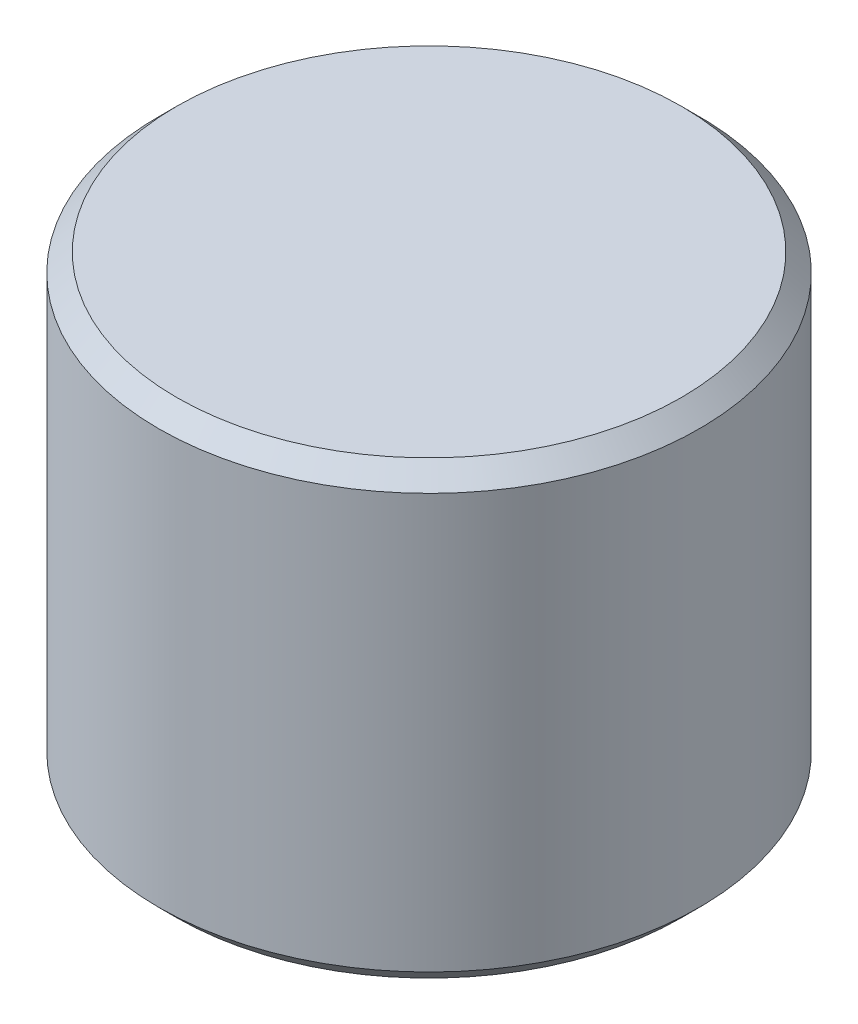
from build123d import *

# Parameters (mm, degrees)
SKETCH1_R           = 3
BOSS_EXTRUDE1_DEPTH = 5
CHAMFER1_SIZE       = 0.2


with BuildPart() as part:
    # Sketch1 → Boss-Extrude1 (new body)
    with BuildSketch(Plane(origin=(0, 0, 0), x_dir=(1, 0, 0), z_dir=(0, 1, 0))):
        with Locations(Location((0, 0, 0), (0, 0, 270))):
            Circle(SKETCH1_R)
    extrude(amount=BOSS_EXTRUDE1_DEPTH)

    # Chamfer1
    chamfer1_edges = [part.edges().sort_by_distance(p)[0] for p in [
        (0, 0, -3),
        (0, 5, -3),
    ]]
    chamfer(chamfer1_edges, length=CHAMFER1_SIZE)


solid = part.part
